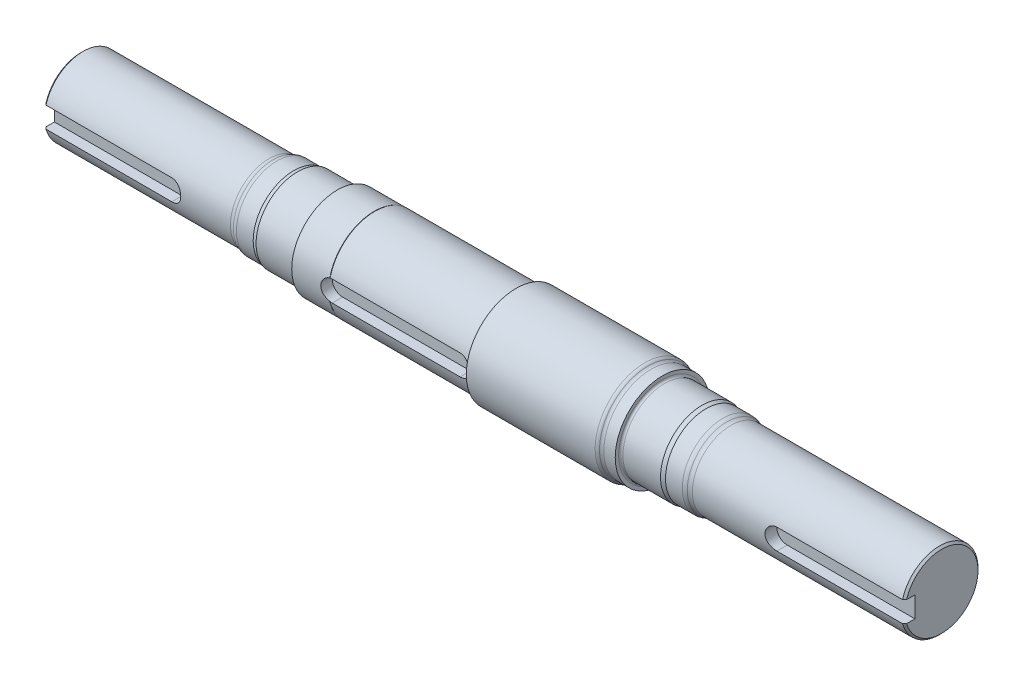
SolidWorks part; units mm, degrees
material "AISI 1045 钢，冷拔"
ref_plane "Front Plane" through (0, 0, 0) normal (0, 0, 1) x (1, 0, 0)
ref_plane "Top Plane" through (0, 0, 0) normal (0, 1, 0) x (1, 0, 0)
ref_plane "Right Plane" through (0, 0, 0) normal (1, 0, 0) x (0, 0, -1)
sketch "Sketch1" plane through (0, 0, 0) normal (0, 0, 1) x (1, 0, 0)
  line L0 (0, 0) -> (1314.45, 0) construction
  line L1 (0, 0) -> (0, 58.7375)
  line L2 (448.564, -69.8627) -> (664.591, -69.8627) construction
  line L3 (448.564, -69.6976) -> (448.564, -69.8627) construction
  line L4 (391.541, -69.6976) -> (448.564, -69.6976) construction
  line L5 (391.541, -63.519) -> (391.541, -69.6976) construction
  line L6 (0, 58.7375) -> (286.9676, 58.7375)
  line L7 (293.116, 58.7375) -> (293.116, 61.9125) construction
  line L8 (299.2644, 61.9125) -> (324.866, 61.9125)
  line L9 (324.866, 61.9125) -> (330.8617, 63.519)
  line L10 (330.8617, 63.519) -> (391.541, 63.519)
  line L11 (448.564, 69.8627) -> (447.9478, 69.6976)
  line L12 (0, 0) -> (1314.45, 0)
  line L13 (888.0094, 72.0217) -> (888.0094, 63.519)
  line L14 (888.0094, 63.519) -> (948.6887, 63.519)
  line L15 (948.6887, 63.519) -> (954.6844, 61.9125)
  line L16 (954.6844, 61.9125) -> (980.286, 61.9125)
  line L17 (986.4344, 61.9125) -> (986.4344, 58.7375) construction
  line L18 (992.5828, 58.7375) -> (1314.45, 58.7375)
  line L19 (1314.45, 58.7375) -> (1314.45, 0)
  line L20 (866.013, 72.0217) -> (866.013, 76.073) construction
  line L21 (861.363, 76.073) -> (664.591, 76.073)
  line L22 (664.591, 76.073) -> (664.591, 69.8627)
  line L23 (870.663, 72.0217) -> (888.0094, 72.0217)
  line L24 (391.541, 63.519) -> (391.541, 69.6976)
  line L25 (391.541, 69.6976) -> (447.9478, 69.6976)
  line L27 (448.564, 69.8627) -> (664.591, 69.8627)
  line L28 (866.013, -72.0217) -> (888.0094, -72.0217) construction
  line L29 (664.591, -76.073) -> (664.591, -69.8627) construction
  line L30 (866.013, -76.073) -> (664.591, -76.073) construction
  line L31 (866.013, -72.0217) -> (866.013, -76.073) construction
  line L32 (986.4344, -58.7375) -> (1314.45, -58.7375) construction
  line L33 (986.4344, -61.9125) -> (986.4344, -58.7375) construction
  line L34 (954.6844, -61.9125) -> (986.4344, -61.9125) construction
  line L35 (948.6887, -63.519) -> (954.6844, -61.9125) construction
  line L36 (888.0094, -63.519) -> (948.6887, -63.519) construction
  line L37 (888.0094, -72.0217) -> (888.0094, -63.519) construction
  line L40 (330.8617, -63.519) -> (391.541, -63.519) construction
  line L41 (324.866, -61.9125) -> (330.8617, -63.519) construction
  line L42 (293.116, -61.9125) -> (324.866, -61.9125) construction
  line L43 (293.116, -58.7375) -> (293.116, -61.9125) construction
  line L44 (0, -58.7375) -> (293.116, -58.7375) construction
  arc A0 (980.286, 61.9125) -> (986.4344, 60.325) centre (980.286, 49.2125) cw
  arc A1 (986.4344, 60.325) -> (992.5828, 58.7375) centre (992.5828, 71.4375) ccw
  arc A2 (870.663, 72.0217) -> (866.013, 74.0473) centre (870.663, 78.3717) cw
  arc A3 (861.363, 76.073) -> (866.013, 74.0473) centre (861.363, 69.723) cw
  arc A4 (293.116, 60.325) -> (299.2644, 61.9125) centre (299.2644, 49.2125) cw
  arc A5 (293.116, 60.325) -> (286.9676, 58.7375) centre (286.9676, 71.4375) cw
  dimension "D25" = 12.7
  dimension "D26" = 6.35
  dimension "D27" = 12.7
  dimension "D1" = 1314.45
  dimension "D2" = 328.0156
  dimension "D3" = 98.425
  dimension "D4" = 66.675
  dimension "D5" = 15
  dimension "D6" = 21.9964
  dimension "D7" = 664.591
  dimension "D8" = 448.564
  dimension "D9" = 391.541
  dimension "D10" = 66.675
  dimension "D11" = 98.425
  dimension "D12" = 496.4684
  dimension "D13" = 152.146
  dimension "D14" = 139.7254
  dimension "D15" = 117.475
  dimension "D16" = 123.825
  dimension "D17" = 127.0381
  dimension "D18" = 15
  dimension "D19" = 139.3952
  dimension "D20" = 144.0434
  dimension "D21" = 127.0381
  dimension "D22" = 123.825
  dimension "D23" = 117.475
  dimension "D24" = 15
revolve "Revolve1" add sketch "Sketch1" angle 360 about L12
fillet "Fillet3" radius 3.302 2 edges at (888.0094, 0, 63.519) (391.541, 0, 63.519)
fillet "Fillet4" radius 1.524 1 edges at (664.591, 0, 69.8627)
chamfer "Chamfer1" distance 3.048 angle 45 2 edges at (1314.45, 0, 58.7375) (0, 0, 58.7375)
sketch "Sketch2" plane through (0, 0, 0) normal (0, 0, 1) x (1, 0, 0)
  line L0 (0, 15.875) -> (195.199, 15.875)
  line L1 (0, 55.6895) -> (0, -55.6895) construction
  line L2 (0, 0) -> (1314.45, 0) construction
  line L3 (0, -15.875) -> (195.199, -15.875)
  line L4 (0, 15.875) -> (0, -15.875)
  line L5 (1314.45, -55.6895) -> (1314.45, 55.6895) construction
  line L6 (1314.45, -55.6895) -> (1314.45, 55.6895) construction
  line L7 (657.225, 0) -> (657.225, 199.1107) construction
  line L8 (1314.45, 15.875) -> (1314.45, -15.875)
  line L9 (1314.45, -15.875) -> (1119.251, -15.875)
  line L10 (1314.45, 15.875) -> (1119.251, 15.875)
  arc A0 (195.199, 15.875) -> (195.199, -15.875) centre (195.199, 0) cw
  arc A1 (1119.251, 15.875) -> (1119.251, -15.875) centre (1119.251, 0) ccw
  dimension "D2" = 195.199
  dimension "D1" = 31.75
extrude "Extrude1" cut sketch "Sketch2" along normal through all from offset 40.6766
sketch "Sketch3" plane through (0, 0, 0) normal (0, 0, 1) x (1, 0, 0)
  line L0 (0, 0) -> (647.101, 0) construction
  line L1 (451.739, -15.875) -> (647.101, -15.875)
  line L2 (451.739, 15.875) -> (647.101, 15.875)
  line L4 (0, 15.875) -> (647.101, 15.875) construction
  line L5 (0, -15.875) -> (647.101, -15.875) construction
  arc A0 (647.101, 15.875) -> (647.101, -15.875) centre (647.101, 0) cw
  arc A1 (451.739, 15.875) -> (451.739, -15.875) centre (451.739, 0) ccw
  dimension "D1" = 31.75
  dimension "D2" = 451.739
  dimension "D3" = 195.362
extrude "Extrude2" cut sketch "Sketch3" along normal through all from offset 52.1601
